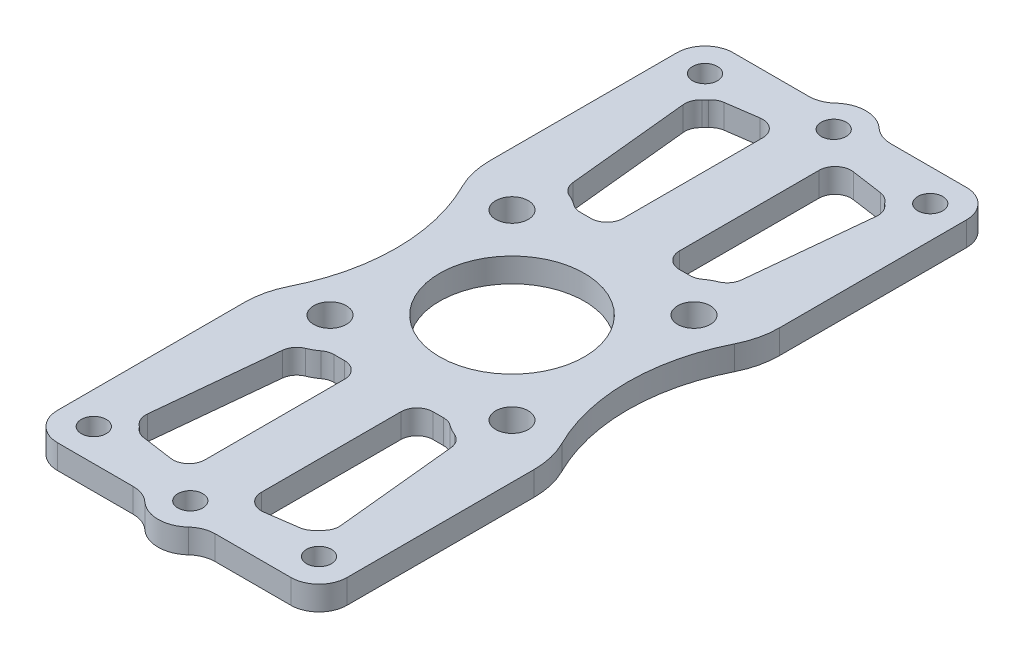
from build123d import *

# Parameters (mm, degrees)
SKETCH_3_R          = 1.55
SKETCH_3_R_2        = 2.025
SKETCH_3_R_3        = 9
EXTRUDE_1_DEPTH     = 3
CUT_EXTRUDE_2_DEPTH = 3
FILLET_3_R          = 2
FILLET_4_R          = 3.5
FILLET_5_R          = 10


with BuildPart() as part:
    # 草图3 → 凸台-拉伸1 (new body)
    with BuildSketch(Plane(origin=(0, 0, 0), x_dir=(1, 0, 0), z_dir=(0, 1, 0))):
        with BuildLine():
            Line((-18, -12.649110641), (-18, -42))
            Line((-18, -42), (-3.464101615, -42))
            ThreePointArc((-3.464101615, -42), (0, -44), (3.464101615, -42))
            Line((3.464101615, -42), (18, -42))
            Line((18, -42), (18, -12.649110641))
            ThreePointArc((18, -12.649110641), (14.396078054, 0), (18, 12.649110641))
            Line((18, 12.649110641), (18, 42))
            Line((18, 42), (3.464101615, 42))
            ThreePointArc((3.464101615, 42), (0, 44), (-3.464101615, 42))
            Line((-3.464101615, 42), (-18, 42))
            Line((-18, 42), (-18, 12.649110641))
            ThreePointArc((-18, 12.649110641), (-14.396078054, 0), (-18, -12.649110641))
        make_face()
        with Locations(Location((-14, -38, 0), (0, 0, 270))):
            Circle(SKETCH_3_R, mode=Mode.SUBTRACT)
        with Locations(Location((-11.313708499, -11.313708499, 0), (0, 0, 270))):
            Circle(SKETCH_3_R_2, mode=Mode.SUBTRACT)
        with Locations(Location((14, -38, 0), (0, 0, 270))):
            Circle(SKETCH_3_R, mode=Mode.SUBTRACT)
        with Locations(Location((11.313708499, -11.313708499, 0), (0, 0, 270))):
            Circle(SKETCH_3_R_2, mode=Mode.SUBTRACT)
        with Locations(Location((-11.313708499, 11.313708499, 0), (0, 0, 270))):
            Circle(SKETCH_3_R_2, mode=Mode.SUBTRACT)
        with Locations(Location((-14, 38, 0), (0, 0, 270))):
            Circle(SKETCH_3_R, mode=Mode.SUBTRACT)
        with Locations(Location((0, 0, 0), (0, 0, 270))):
            Circle(SKETCH_3_R_3, mode=Mode.SUBTRACT)
        with Locations(Location((11.313708499, 11.313708499, 0), (0, 0, 270))):
            Circle(SKETCH_3_R_2, mode=Mode.SUBTRACT)
        with Locations(Location((14, 38, 0), (0, 0, 270))):
            Circle(SKETCH_3_R, mode=Mode.SUBTRACT)
        with Locations(Location((0, -40, 0), (0, 0, 270))):
            Circle(SKETCH_3_R, mode=Mode.SUBTRACT)
        with Locations(Location((0, 40, 0), (0, 0, 270))):
            Circle(SKETCH_3_R, mode=Mode.SUBTRACT)
    extrude(amount=EXTRUDE_1_DEPTH)

    # 草图8 → 切除-拉伸2 (cut)
    with BuildSketch(Plane(origin=(0, 3, 0), x_dir=(1, 0, 0), z_dir=(0, 1, 0))):
        with BuildLine():
            Line((-3.5, 36.974618639), (-10.555330306, 35.966714309))
            ThreePointArc((-10.555330306, 35.966714309), (-11.241007094, 35.103802813), (-12.136155057, 34.46077946))
            Line((-12.136155057, 34.46077946), (-10.351224988, 16.728837813))
            ThreePointArc((-10.351224988, 16.728837813), (-8.841586099, 16.226814527), (-7.538791281, 15.313708499))
            Line((-7.538791281, 15.313708499), (-3.5, 15.313708499))
            Line((-3.5, 15.313708499), (-3.5, 36.974618639))
        make_face()
        with BuildLine():
            Line((3.5, 36.974618639), (3.5, 15.313708499))
            Line((3.5, 15.313708499), (7.538791281, 15.313708499))
            ThreePointArc((7.538791281, 15.313708499), (8.841586099, 16.226814527), (10.351224988, 16.728837813))
            Line((10.351224988, 16.728837813), (12.136155057, 34.46077946))
            ThreePointArc((12.136155057, 34.46077946), (11.241007094, 35.103802813), (10.555330306, 35.966714309))
            Line((10.555330306, 35.966714309), (3.5, 36.974618639))
        make_face()
        with BuildLine():
            Line((3.5, -36.974618639), (10.555330306, -35.966714309))
            ThreePointArc((10.555330306, -35.966714309), (11.241007094, -35.103802813), (12.136155057, -34.46077946))
            Line((12.136155057, -34.46077946), (10.351224988, -16.728837813))
            ThreePointArc((10.351224988, -16.728837813), (8.841586099, -16.226814527), (7.538791281, -15.313708499))
            Line((7.538791281, -15.313708499), (3.5, -15.313708499))
            Line((3.5, -15.313708499), (3.5, -36.974618639))
        make_face()
        with BuildLine():
            Line((-10.555330306, -35.966714309), (-3.5, -36.974618639))
            Line((-3.5, -36.974618639), (-3.5, -15.313708499))
            Line((-3.5, -15.313708499), (-7.538791281, -15.313708499))
            ThreePointArc((-7.538791281, -15.313708499), (-8.841586099, -16.226814527), (-10.351224988, -16.728837813))
            Line((-10.351224988, -16.728837813), (-12.136155057, -34.46077946))
            ThreePointArc((-12.136155057, -34.46077946), (-11.241007094, -35.103802813), (-10.555330306, -35.966714309))
        make_face()
    extrude(amount=-CUT_EXTRUDE_2_DEPTH, mode=Mode.SUBTRACT)

    # 圆角3
    fillet_3_edges = [part.edges().sort_by_distance(p)[0] for p in [
        (7.538791281, 1.5, -15.313708499),
        (3.5, 1.5, -15.313708499),
        (3.5, 1.5, -36.974618639),
        (10.555330306, 1.5, -35.966714309),
        (12.136155057, 1.5, -34.46077946),
        (-10.351224988, 1.5, 16.728837813),
        (-7.538791281, 1.5, 15.313708499),
        (-3.5, 1.5, 15.313708499),
        (-3.5, 1.5, 36.974618639),
        (-10.555330306, 1.5, 35.966714309),
        (-12.136155057, 1.5, 34.46077946),
        (7.538791281, 1.5, 15.313708499),
        (10.351224988, 1.5, 16.728837813),
        (12.136155057, 1.5, 34.46077946),
        (10.555330306, 1.5, 35.966714309),
        (3.5, 1.5, 36.974618639),
        (3.5, 1.5, 15.313708499),
        (-7.538791281, 1.5, -15.313708499),
        (-10.351224988, 1.5, -16.728837813),
        (-12.136155057, 1.5, -34.46077946),
        (-10.555330306, 1.5, -35.966714309),
        (-3.5, 1.5, -36.974618639),
        (-3.5, 1.5, -15.313708499),
        (10.351224988, 1.5, -16.728837813),
    ]]
    fillet(fillet_3_edges, radius=FILLET_3_R)

    # 圆角4
    fillet_4_edges = [part.edges().sort_by_distance(p)[0] for p in [
        (-18, 1.5, 42),
        (-18, 1.5, -42),
        (-3.464101615, 1.5, -42),
        (3.464101615, 1.5, -42),
        (18, 1.5, -42),
        (18, 1.5, 42),
        (3.464101615, 1.5, 42),
        (-3.464101615, 1.5, 42),
    ]]
    fillet(fillet_4_edges, radius=FILLET_4_R)

    # 圆角5
    fillet_5_edges = [part.edges().sort_by_distance(p)[0] for p in [
        (-18, 1.5, 12.649110641),
        (-18, 1.5, -12.649110641),
        (18, 1.5, -12.649110641),
        (18, 1.5, 12.649110641),
    ]]
    fillet(fillet_5_edges, radius=FILLET_5_R)


solid = part.part
